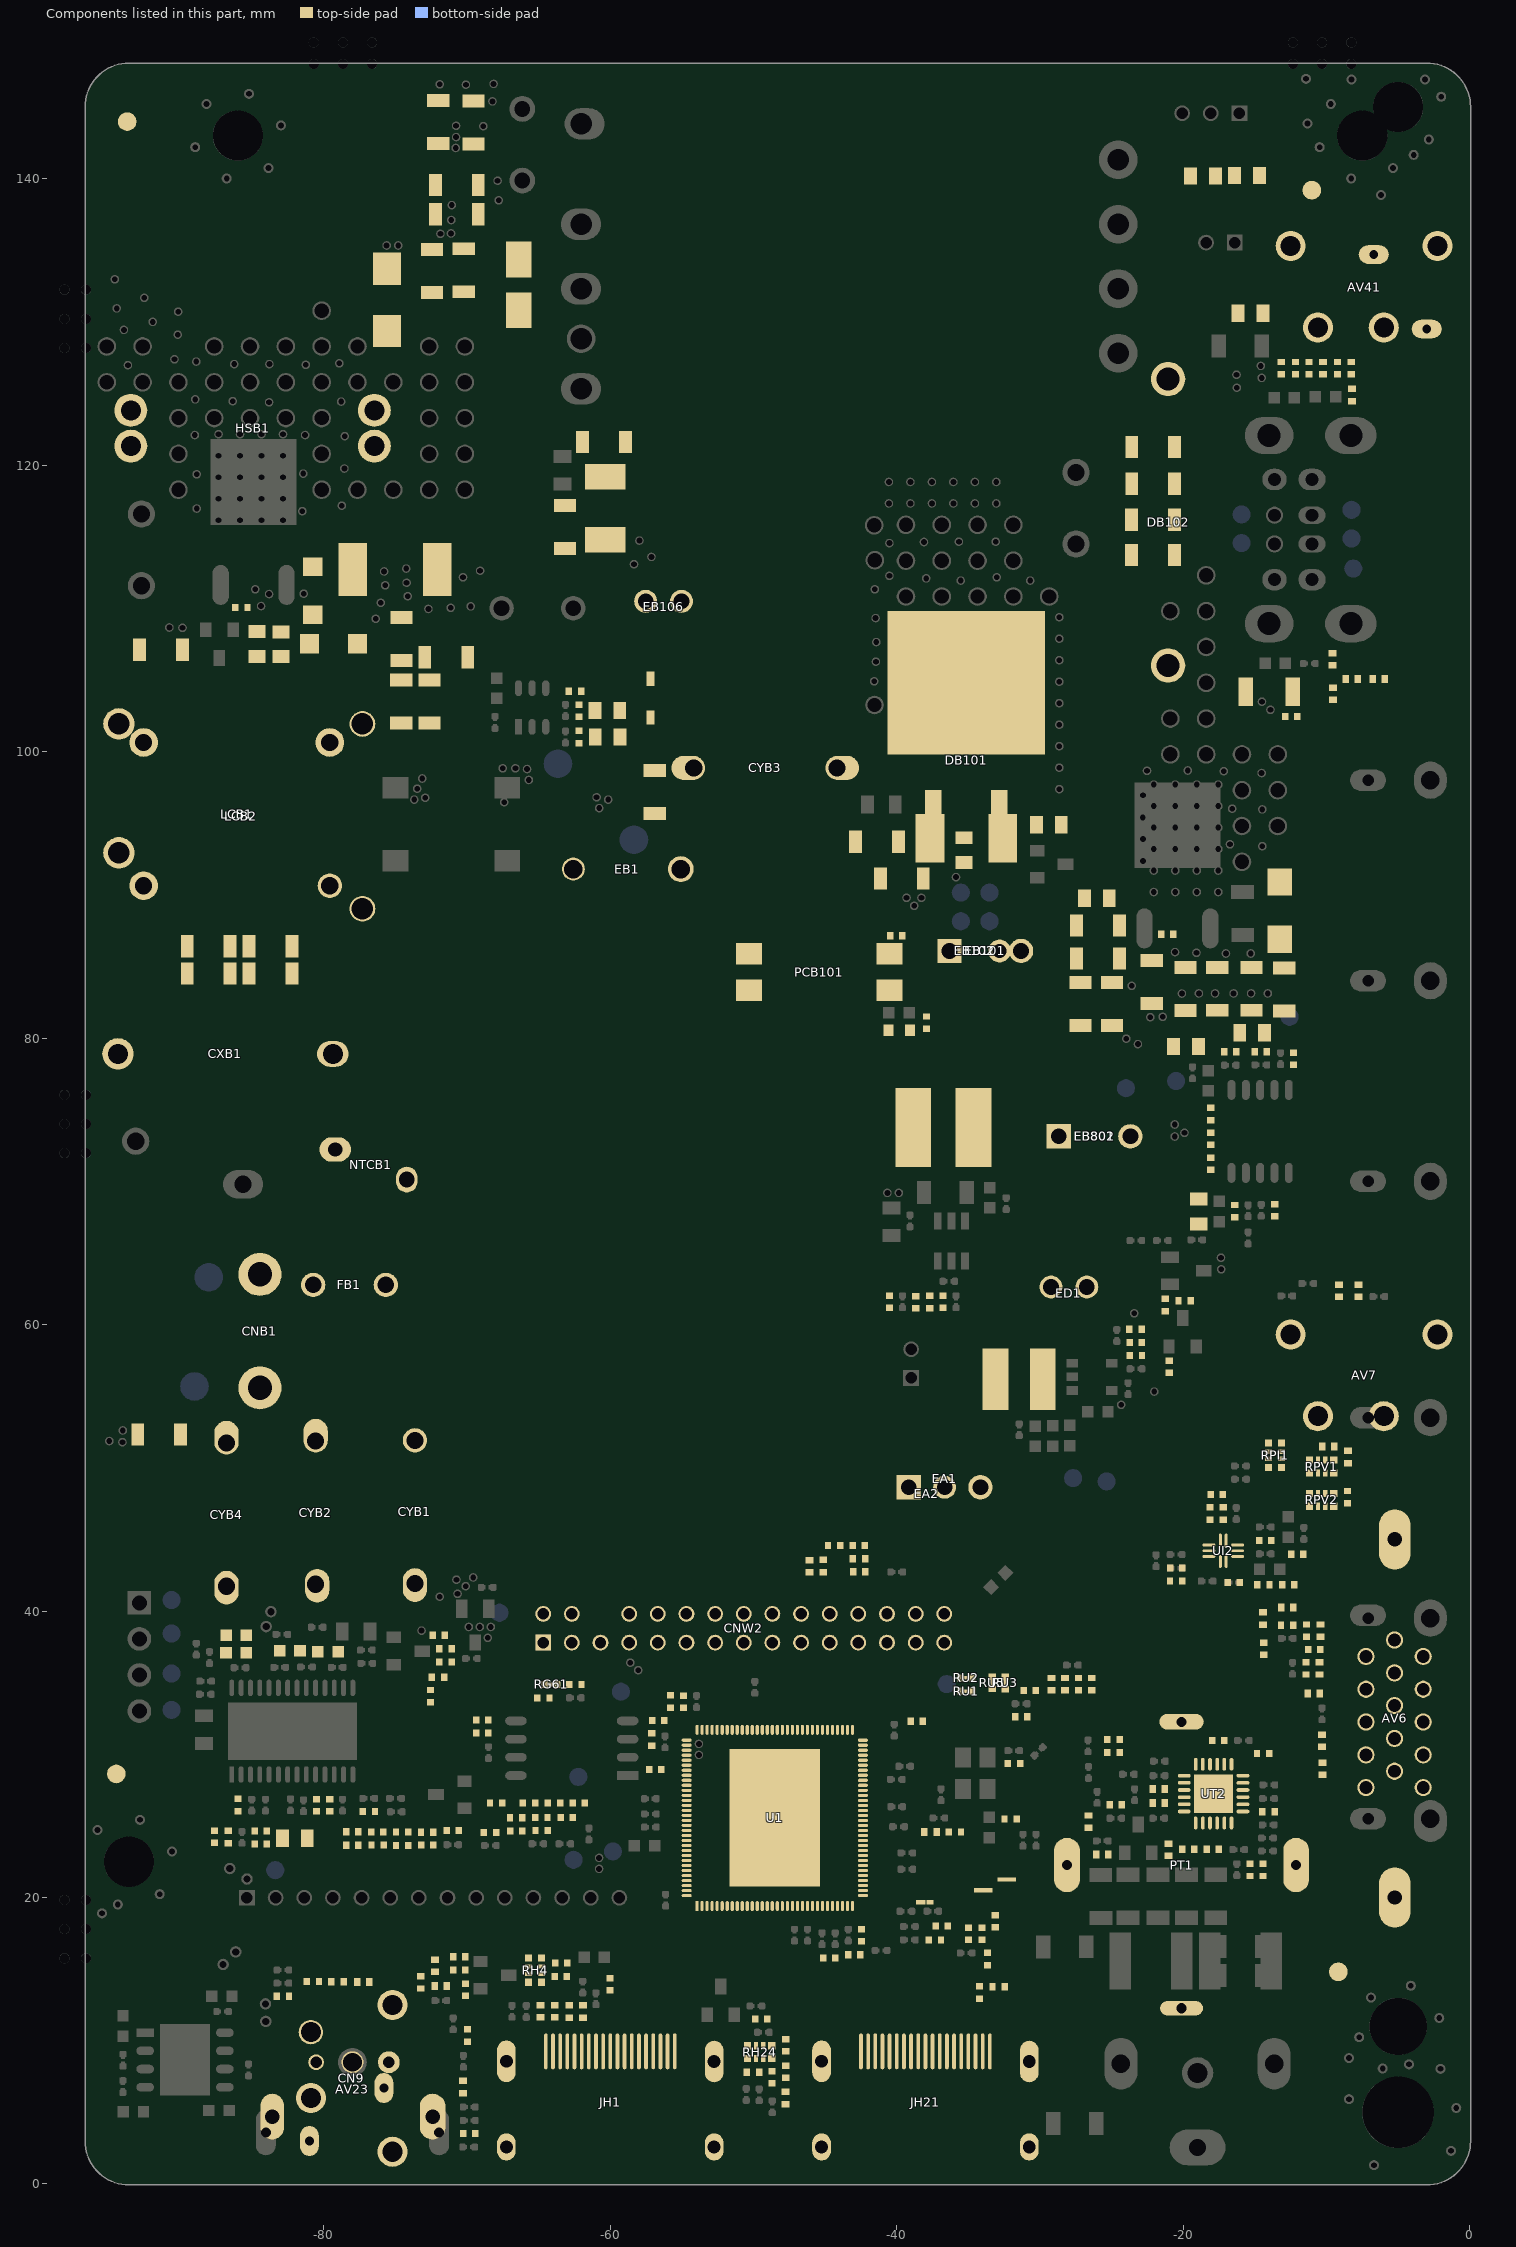
[diagram p0: the components of this part, seen from the top]
# Altium PCB MISC86372.PcbDoc (part 4 of 16)
Units mm, origin at the board's own origin, x right, y up, seen from the top; angles counter-clockwise.
Board outline 96.73 x 148.13 mm, 2 copper layers (TopLayer, BottomLayer), stack 1.571 mm thick; 578 components, 318 nets, 2702 pads, 836 vias.

## Footprints (in the part's own frame and the unit in brackets; to place one, negate y for a bottom-side part, rotate by r counter-clockwise, add the part's x,y. Pads: shape width x height; smd on the part's side, far side on the other; paste and mask are expansions set on the pad) (continued)
CAP13*5-V-10-1#1 [mm] "Walsin;YU1AH471M060DAMD0H;160718（18.03.15  更新孔径）"
  round 1.7 hole 1.2: 1(-5,0)
  oval 2.35x1.7 hole 1.2 copper offset 0.1,0: 2(5,0)
  oval 2.55x1.9 on Top Overlay: 61(-5,0) 61(5,0)
  silkscreen extent -5.71,-3 5.81,3
CAP13*5-V-10-1#2 [mm] "Walsin;YU1AH471M060DAMD0H;160718（18.03.15  更新孔径）"
  oval 2.35x1.7 hole 1.2 copper offset -0.375,0: 1(-5,0)
  oval 2.35x1.7 hole 1.2 copper offset 0.1,0.1: 2(5,0)
  oval 2.55x1.9 on Top Overlay: 61(-5,0) 61(5,0)
  silkscreen extent -5.71,-3 5.81,3
CAP13*5-V-10-1#3 [mm] "Walsin;YU1AH471M060DAMD0H;160718（18.03.15  更新孔径）"
  oval 2.35x1.7 hole 1.2 copper offset -0.375,0: 1(-5,0)
  oval 2.35x1.7 hole 1.2 copper offset 0.375,0: 2(5,0)
  oval 2.55x1.9 on Top Overlay: 61(-5,0) 61(5,0)
  silkscreen extent -5.71,-3 5.81,3
CAP13*5-V-10-1#4 [mm] "Walsin;YU1AH471M060DAMD0H;160718（18.03.15  更新孔径）"
  oval 2.35x1.7 hole 1.2 copper offset -0.375,0: 1(-5,0)
  oval 2.35x1.7 hole 1.2 copper offset 0.1,0: 2(5,0)
  oval 2.55x1.9 on Top Overlay: 61(-5,0) 61(5,0)
  silkscreen extent -5.71,-3 5.81,3
CAP18*8.5-V-15 [mm] "PX334K3ID49H200D9R(凯励)(18.01.12更新孔径）(18.07.18 更新丝印框，加了公差）"
  oval 2.2x1.8 hole 1.4: 1(-7.5,0)
  round 2.2 hole 1.4: 2(7.5,0)
  round 2.4 on Top Overlay: 77(7.5,0) 78(-7.5,0)
  silkscreen extent -9.25,-4.45 9.25,4.45
CAUTION [mm]
  silkscreen extent -10.17,-3.72 12.33,4.08
COLD [mm]
CON2-H7.92 [mm] "因物料底部露金属，20170630增加1.8mm安规禁布"
  round 3 / inner round 3 / far side round 4 hole 1.7: 1(0,3.96)
  round 3 / inner round 3 / far side round 4.4 hole 1.7: 3(0,-3.96)
  round 3.2 on Top Overlay: 109(0,3.96) 110(0,-3.96)
  silkscreen extent -12,-5.94 4.23,5.94, body extent -11.46,-6.04 0.56,5.86, height 8.49
"Conformal Coating" [mm] "三防漆虚线框"
  round 0.3 on Mech2: 0(0,0)
CQC [mm]
D2PAK3 [mm] "伟达电子；SFS1006G;增加TO-252兼容；160309"
  oval 2.794x1.143 smd: 1(5.542,-2.2) 3(5.542,2.4)
  rect 2.794x1.143 smd: 1(5.544,-2.2) 3(5.544,2.4)
  rect 3.4x2 smd paste-5 mask-5: 1(7.494,-2.44) 3(7.494,2.64)
  rect 10x11 smd paste-11 mask-11: 2(-3.356,0.1)
  rect 6x6 smd paste-10 mask-11: 2(-2.158,0.1)
  TopLayer pour cut-out: 3.373,2.4 6.497,2.4 6.497,-2.245 6.438,-2.54 6.271,-2.791 6.02,-2.958 5.725,-3.017 5.725,-3.017 5.725,-2.199 4.141,-2.199 4.141,-3.024 3.847,-2.966 3.598,-2.799 3.432,-2.55 3.373,-2.256 3.373,-2.256
  silkscreen extent -9.13,-5.69 4.84,5.89, body extent -6.91,-5.15 8.79,5.35, height 4.7
D3-H-20 [mm] "肖特基二极管"
  round 2.6 on Top Overlay: 0(10,0) 1(-10,0)
  round 2.4 hole 1.6: A(-10,0) K(10,0)
  silkscreen extent -13,-2.6 13,2.6, body extent -12.62,-2.69 12.63,2.69, height 11.81
DB15-HF-1 [mm] "兴万联电子：WLHD-051A"
  oval 4.4x2.4 on Top Overlay: 0(-12.5,5.227) 0(12.5,5.227)
  round 1.2 hole 0.9: 1(4.33,7.247) 2(2.04,7.247) 3(-0.25,7.247) 4(-2.54,7.247) 5(-4.83,7.247) 6(5.475,5.247) 7(3.185,5.247) 8(0.895,5.247) 9(-1.395,5.247) 10(-3.685,5.247) 11(4.33,3.247) 12(2.04,3.247) 13(-0.25,3.247) 14(-2.54,3.247) 15(-4.83,3.247)
  oval 4.2x2.2 hole 1 slot 3 at 0 deg: 16(-12.5,5.227) 17(12.5,5.227)
  round 1.5 on Top Overlay: 30(-4.83,3.247) 31(-2.54,3.247) 32(-0.25,3.247) 33(2.04,3.247) 34(4.33,3.247) 35(5.475,5.247) 36(3.185,5.247) 37(0.895,5.247) 38(-1.395,5.247) 39(-3.685,5.247) 40(-4.83,7.247) 41(-2.54,7.247) 42(-0.25,7.247) 43(2.04,7.247) 44(4.33,7.247)
  BottomLayer pour cut-out: -4.814,8.609 -4.814,5.885 -4.587,5.885 -4.443,5.742 -3.456,5.742 -3.175,5.461 -3.175,5.029 -3.454,4.75 -4.42,4.75 -4.56,4.609 -4.797,4.609 -4.83,4.576 -4.83,1.885 4.33,1.885 4.33,3.247 4.298,3.279 4.298,4.609 4.105,4.609 3.95,4.764 2.44,4.764 2.285,4.609 1.817,4.609 1.664,4.763 0.648,4.763 0.368,5.042 0.368,5.474 0.622,5.728 1.651,5.728 1.803,5.88 2.286,5.88 2.438,5.728 3.95,5.728 4.107,5.885 4.33,5.885 4.33,8.609
  silkscreen extent -15.59,0 15.59,9.48, body extent -16.75,-62.85 16.75,8.75, height 14.13
DIODE-S0402 [mm] "DVD上使用的ESD"
  rect 0.45x0.55 smd mask+0.051: A(-0.425,0) K(0.425,0)
  silkscreen extent -0.8,-0.43 0.91,0.43, body extent -0.5,-0.25 0.5,0.25, height 0.5
DIODE-S-2 [mm] "1N5819-SMA;170509去除兼容,20180607减少内距0.4mm以兼容SMAF"
  rect 1.8x2.8 smd: A(-2.2,0) K(2.2,0)
  silkscreen extent -3.5,-1.6 3.7,1.61, body extent -2.6,-1.4 2.6,1.4, height 1.91
DIODE-S-12 [mm] "Formosa MS ;BAV19WS THRU BAV21WS/PMEG2010BEA(高度为1.1mm)"
  rect 1x0.55 smd: A(1.35,0) K(-1.35,0)
  silkscreen extent -0.9,-0.67 0.9,0.67, body extent -1.35,-0.63 1.35,0.63, height 1
DIODE-S-14 [mm] "ROHM;FSL14"
  rect 1.3x1.35 smd: A(1.675,0) K(-1.675,0)
  silkscreen extent -1.55,-1 1.55,1, body extent -1.95,-1 1.95,1, height 1.08
DIODE-SMA-1 [mm] "SUF103A(SECOS);14.06.13"
  rect 1.9x1.7 smd: A(-2,0) K(2,0)
  silkscreen extent -2.3,-1.45 2.3,1.45, body extent -2.64,-1.45 2.64,1.45, height 2.44
DIODE-SMA-2 [mm] "LITE-ON,SMAJ20A,0710_2018"
  rect 2.25x1.95 smd mask+0.051: A(-2.17,0) K(2.17,0)
  silkscreen extent -2.27,-1.46 2.3,1.46, body extent -2.59,-1.46 2.62,1.46, height 2.4
DOLBY-SILK [mm]
  silkscreen extent -0.4,-4.5 36.6,5
EC(5*11)-V-2.5 [mm] "机插2.5间距"
  round 1.8 on Top Overlay: 0(-1.25,0) 0(1.25,0)
  round 0.5 on Keep-Out: 0(0,-0.787)
  round 1.6 hole 1.1: 1(-1.25,0) 2(1.25,0)
  BottomLayer lines w0.6: -1.64,-0.31 -2.806,1.556 ; -1.25,0 -2.806,1.556 ; -0.94,0.39 -2.806,1.556 ; 0.94,-0.39 2.806,-1.556 ; 1.25,0 2.806,-1.556 ; 1.64,0.31 2.806,-1.556
  silkscreen extent -2.75,-2.75 3,2.75, body extent -2.48,-2.52 2.5,2.47, height 12.5
EC(6.3*11)-V-2.5#1 [mm] "机插2.5间距"
  round 0.5 on Keep-Out: 0(0,-0.889)
  round 1.6 hole 1.1: 1(-1.25,0) 2(1.25,0)
  round 1.8 on Top Overlay: 5(1.25,0) 6(-1.25,0)
  BottomLayer lines w0.6: -1.665,-0.275 -1.681,-0.244 -1.691,-0.225 ; -1.25,0 -1.417,0.2 -2.279,1.227 -2.664,1.685 ; -0.907,0.361 -0.952,0.395 ; 0.907,-0.361 2.664,-1.685 ; 1.25,0 2.664,-1.685 ; 1.665,0.275 2.664,-1.685 ; -2.664,1.685 -2.501,1.365 -2.382,1.132 ; -2.664,1.685 -1.159,0.551 -0.969,0.408 -0.952,0.395 ; -2.382,1.132 -2.382,1.132 ; -2.382,1.132 -1.805,0 -1.804,-0.003 -1.691,-0.225 ; -1.691,-0.225 -1.691,-0.225 ; -1.691,-0.225 -1.691,-0.225 ; -1.691,-0.225 -1.691,-0.225 ; -1.691,-0.225 -1.691,-0.225 ; -1.691,-0.225 -1.691,-0.225 ; -1.691,-0.225 -1.691,-0.225 ; -1.691,-0.225 -1.691,-0.225 ; -1.691,-0.225 -1.691,-0.225 ; -0.952,0.395 -0.952,0.395 ; -0.952,0.395 -0.952,0.395 ; -0.952,0.395 -0.952,0.395 ; -0.952,0.395 -0.952,0.395 ; -0.952,0.395 -0.952,0.395
  silkscreen extent -3.17,-3.17 3.51,3.17, body extent -3,-3 2.98,2.99, height 12.5
EC(6.3*11)-V-2.5#2 [mm] "机插2.5间距"
  round 0.5 on Keep-Out: 0(0,-0.889)
  round 1.6 hole 1.1: 1(-1.25,0) 2(1.25,0)
  round 1.8 on Top Overlay: 5(1.25,0) 6(-1.25,0)
  BottomLayer lines w0.6: -1.665,-0.275 -1.691,-0.225 -2.664,1.685 ; -1.25,0 -2.664,1.685 ; -0.907,0.361 -0.952,0.395 ; 0.907,-0.361 2.664,-1.685 ; 1.25,0 2.664,-1.685 ; 1.665,0.275 2.664,-1.685 ; -2.664,1.685 -1.25,0.62 -0.952,0.395 ; -0.952,0.395 -0.952,0.395 ; -0.952,0.395 -0.952,0.395 ; -0.952,0.395 -0.952,0.395
  silkscreen extent -3.17,-3.17 3.51,3.17, body extent -3,-3 2.98,2.99, height 12.5
EC(8*11)-V-3.5 [mm]
  rect 1.6x1.6 hole 1: 1(-1.75,0)
  rect 1.8x1.8 on Top Overlay: 1(-1.75,0)
  round 1.8 on Top Overlay: 1(1.75,0)
  round 1.6 hole 1: 2(1.75,0)
  silkscreen extent -4.25,-4.25 4.45,4.25, body extent -3.98,-3.98 4.01,4.01, height 12.51
EC(10*12)-V-5 [mm] "机插5间距"
  rect 1.9x1.9 on Top Overlay: 0(-2.5,0)
  round 0.5 on Keep-Out: 0(-1.01,1.193)
  round 1.9 on Top Overlay: 0(2.5,0)
  rect 1.7x1.7 hole 1.1: 1(-2.5,0)
  round 1.7 hole 1.1: 2(2.5,0)
  BottomLayer lines w0.6: -2.89,-0.31 -2.92,-0.262 ; -2.5,0 -2.685,0.185 -3.632,1.132 -4.056,1.556 ; -2.19,0.39 -2.219,0.408 -2.238,0.42 ; 2.19,-0.39 2.238,-0.42 4.056,-1.556 ; 2.5,0 4.056,-1.556 ; 2.89,0.31 2.92,0.262 4.056,-1.556 ; -4.056,1.556 -4.056,1.556 ; -4.056,1.556 -4.056,1.556 ; -4.056,1.556 -3.321,0.38 -3.084,0 -3.055,-0.046 -2.931,-0.244 -2.92,-0.262 ; -4.056,1.556 -3.751,1.365 -3.529,1.227 -2.454,0.555 -2.238,0.42 ; -4.056,1.556 -4.056,1.556 ; -2.92,-0.262 -2.92,-0.262 ; -2.92,-0.262 -2.92,-0.262 ; -2.92,-0.262 -2.92,-0.262 ; -2.238,0.42 -2.238,0.42
  silkscreen extent -5.25,-5.25 5.57,5.25, body extent -4.98,-4.99 5.01,4.99, height 12.01
EC(10*12.5)-V-5#1 [mm] "机插5间距"
  round 0.5 on Keep-Out: 0(-0.75,0)
  rect 1.7x1.7 hole 1.1: 1(-2.5,0)
  rect 1.9x1.9 on Top Overlay: 1(-2.5,0)
  round 1.9 on Top Overlay: 1(2.5,0)
  round 1.7 hole 1.1: 2(2.5,0)
  BottomLayer lines w0.6: -2.89,-0.31 -2.92,-0.262 ; -2.5,0 -2.749,0.249 -2.815,0.315 -2.994,0.494 -3.084,0.584 -3.315,0.815 -4.056,1.556 ; -2.19,0.39 -2.238,0.42 ; 2.19,-0.39 2.238,-0.42 ; 2.5,0 2.92,-0.42 4.056,-1.556 ; 2.89,0.31 2.92,0.262 ; -4.056,1.556 -3.977,1.507 -3.315,1.093 -2.863,0.81 -2.749,0.739 -2.672,0.691 -2.606,0.65 -2.528,0.601 ; -4.056,1.556 -3.448,0.584 -3.322,0.381 -3.198,0.183 -3.15,0.106 -3.101,0.028 ; -4.056,1.556 -4.056,1.556 ; -3.101,0.028 -3.101,0.028 ; -3.101,0.028 -2.92,-0.262 ; -2.92,-0.262 -2.92,-0.262 ; -2.92,-0.262 -2.92,-0.262 ; -2.528,0.601 -2.528,0.601 ; -2.528,0.601 -2.528,0.601 ; -2.528,0.601 -2.528,0.601 ; -2.528,0.601 -2.5,0.584 -2.337,0.482 -2.266,0.437 -2.254,0.43 -2.238,0.42 ; -2.238,0.42 -2.238,0.42 ; -2.238,0.42 -2.238,0.42 ; -2.238,0.42 -2.238,0.42 ; -2.238,0.42 -2.238,0.42 ; -2.238,0.42 -2.238,0.42 ; 2.238,-0.42 2.92,-0.846 4.056,-1.556 ; 2.238,-0.42 2.238,-0.42 ; 2.92,0.262 3.084,0 3.964,-1.408 4.056,-1.556 ; 2.92,0.262 2.92,0.262
  silkscreen extent -5.2,-5.21 5.57,5.21, body extent -4.98,-4.99 5.01,4.99, height 14.01
EC(10*12.5)-V-5#2 [mm] "机插5间距"
  round 0.5 on Keep-Out: 0(-0.75,0)
  rect 1.7x1.7 hole 1.1: 1(-2.5,0)
  rect 1.9x1.9 on Top Overlay: 1(-2.5,0)
  round 1.9 on Top Overlay: 1(2.5,0)
  round 1.7 hole 1.1: 2(2.5,0)
  BottomLayer lines w0.6: -2.89,-0.31 -4.056,1.556 ; -2.5,0 -4.056,1.556 ; -2.19,0.39 -4.056,1.556 ; 2.19,-0.39 2.238,-0.42 ; 2.5,0 4.056,-1.556 ; 2.89,0.31 2.92,0.262 ; 2.238,-0.42 2.238,-0.42 ; 2.238,-0.42 4.056,-1.556 ; 2.92,0.262 2.92,0.262 ; 2.92,0.262 3.075,0.014 4.056,-1.556
  silkscreen extent -5.2,-5.21 5.57,5.21, body extent -4.98,-4.99 5.01,4.99, height 14.01
EC(13*13)-V-5 [mm] "KF330M200I130A00LR;14-09-17"
  round 1.7 hole 1: 1(-2.5,0) 2(2.5,0)
  round 1.9 on Top Overlay mask+0.076: 2(-2.5,0) 3(2.5,0)
  silkscreen extent -6.75,-6.75 7.26,6.75, body extent -6.7,-6.72 6.82,6.75, height 14.51
EC(18*31.5)-H-7.5 [mm] "SAMXON  (18*45),板上高度15.235mm;170320更新开槽"
  round 1.8 / inner rect 2.5x2.5 / far side rect 2.5x2.5 hole 1.3: 1(3.75,0)
  round 1.6 / inner round 2.5 / far side round 2.5 hole 1.3: 2(-3.75,0)
  round 2.7 on Top Overlay: 2(-3.75,0)
  rect 2.7x2.7 on Top Overlay: 2(3.75,0)
  KeepOutLayer lines w0.127: -6.75,-39.5 -6.75,-4.5 6.75,-4.5 6.75,-39.5 -6.75,-39.5
  silkscreen extent -9.26,-38.11 9.25,-1.26
EVA(7*7*3) [mm] "7*7*3"
  silkscreen extent -4.5,-4.5 4.5,4.5
Fixed [mm] "麦拉片塑胶固定柱(4.50×6.49mm-尼龙-白色)"
  round 2.5 on Keep-Out: 0(0,0)
  silkscreen extent -1.9,-1.9 1.9,1.9
FUSE1.1A-S [mm] "保险丝：FSMD005-1206(FUZETEC)（兼容1206F8.00A063V 高度0.8mm），18.03.07）"
  rect 1x2 smd: 1(-1.65,0) 2(1.65,0)
  silkscreen extent -2.4,-1.2 2.4,1.2, body extent -1.75,-0.9 1.75,0.9, height 1
"FUSE8.5*4-V-5(T3.15AL 250V~)" [mm] "SMT1315AP/2010T1A250VA1(编带/华德)"
  round 1.7 hole 1.15: 1(2.54,0) 2(-2.54,0)
  round 1.9 on Top Overlay: 4(2.54,0) 5(-2.54,0)
  BottomLayer lines w1: 2.811,0.228 3.977,-1.437 ; 2.54,0 3.977,-1.437 ; 2.312,-0.271 3.977,-1.437 ; -2.312,0.271 -3.977,1.437 ; -2.54,0 -3.977,1.437 ; -2.811,-0.228 -3.977,1.437
  silkscreen extent -4.3,-2.1 4.3,2.1, body extent -4.3,-2.1 4.3,2.1, height 8.5
GND#1 [mm] "导通线"
  rect 0.5x0.3 smd paste-0.45 mask-0.45: JP_1K(-0.32,0)
  rect 0.66x0.3 smd paste-0.45 mask-0.45: JP_2K(0.32,0)
GND#2 [mm] "导通线"
  rect 0.66x0.3 smd paste-0.45 mask-0.45: JP_1K(-0.32,0) JP_2K(0.32,0)
HDMI-HS-1#1 [mm] "浙江和丰   HHF-14B000-2SA。17.09.25更新钢网;171107更新焊盘露铜位置(18.04.19 更新大脚孔径）"
  rect 2.2x3.8 on Top Paste: 0(-7.75,4.18) 0(7.753,4.183)
  rect 2.2x6 on Top Paste: 0(-7.75,9.355) 0(7.75,9.355)
  oval 0.26x2.5 smd: 1(4.5,11.258) 2(4,11.258) 3(3.5,11.258) 4(3,11.258) 5(2.5,11.258) 6(2,11.258) 7(1.5,11.258) 8(1,11.258) 9(0.5,11.258) 10(0,11.258) 11(-0.5,11.258) 12(-1,11.258) 13(-1.5,11.258) 14(-2,11.258) 15(-2.5,11.258) 16(-3,11.258) 17(-3.5,11.258) 18(-4,11.258) 19(-4.5,11.258)
  oval 1.3x2.9 hole 0.9 slot 2.5 at 90 deg mask+0.076: 20(-7.25,10.565) 22(7.25,10.55)
  oval 1.3x1.9 hole 0.9 slot 1.5 at 90 deg mask+0.076: 21(-7.25,4.59) 23(7.25,4.59)
  silkscreen extent -7.5,2 7.5,12.19, body extent -10.25,-57.68 10.25,12.17, height 8.42
HDMI-HS-1#2 [mm] "浙江和丰   HHF-14B000-2SA。17.09.25更新钢网;171107更新焊盘露铜位置(18.04.19 更新大脚孔径）"
  rect 2.2x3.8 on Top Paste: 0(-7.75,4.18)
  rect 2.2x6 on Top Paste: 0(-7.75,9.355)
  rect 2.2x3.81 on Top Paste: 0(7.75,9.355)
  rect 2.2x2.032 on Top Paste: 0(7.753,4.183)
  oval 0.26x2.5 smd: 1(4.5,11.258) 2(4,11.258) 3(3.5,11.258) 4(3,11.258) 5(2.5,11.258) 6(2,11.258) 7(1.5,11.258) 8(1,11.258) 9(0.5,11.258) 10(0,11.258) 11(-0.5,11.258) 12(-1,11.258) 13(-1.5,11.258) 14(-2,11.258) 15(-2.5,11.258) 16(-3,11.258) 17(-3.5,11.258) 18(-4,11.258) 19(-4.5,11.258)
  oval 1.3x2.9 hole 0.9 slot 2.5 at 90 deg mask+0.076: 20(-7.25,10.565) 22(7.25,10.55)
  oval 1.3x1.9 hole 0.9 slot 1.5 at 90 deg mask+0.076: 21(-7.25,4.59) 23(7.25,4.59)
  silkscreen extent -7.5,2 7.5,12.19, body extent -10.25,-57.68 10.25,12.17, height 8.42
"Heat-Shrinkable Tube" [mm] "收缩前壁厚0.3+-0.05，收缩后壁厚0.6+-0.1"
  round 0.3 on Mech2: 0(0,0)
"High Voltage" [mm]
  silkscreen extent -0.53,-1.52 0.43,1.27
HOT [mm]
HS149-YZ [mm] "17.5×14.5×0.5-本色-Cu-LHD, 18.05.17  取代HS038的验证封装"
  round 2.3 hole 1.4: 1(-8.5,1.25) 2(-8.5,-1.25) 3(8.5,-1.25) 4(8.5,1.25)
  BottomLayer region: 7.983,-1.016 8.999,-1.016 8.999,1.016 7.983,1.016
  BottomLayer region: -9.017,-1.016 -8.001,-1.016 -8.001,1.016 -9.017,1.016
  silkscreen extent -8.5,-2.5 8.5,2.5
HS(14*14*6) [mm] "14×14×06-THD;14.10.21"
  silkscreen extent -7.1,-7.1 7.1,10.57
L0402 [mm] "电感"
  rect 0.45x0.55 smd mask+0.076: 1(-0.425,0) 2(0.425,0)
  silkscreen extent -0.8,-0.42 0.8,0.43, body extent -0.5,-0.25 0.5,0.25, height 0.5
L0603 [mm] "片式磁珠、电感、ESD"
  rect 0.813x0.8 smd mask+0.076: 1(-0.706,0) 2(0.706,0)
  silkscreen extent -1.27,-0.55 1.27,0.55, body extent -0.8,-0.4 0.8,0.4, height 0.8
L(4*3*2.55)-S [mm] "贴片磁珠；SMB -302540-K5B- L1;15.02.05（17.12.07更新高度信息）"
  rect 2.5x1.8 smd: 1(-1.775,0) 2(1.775,0)
  silkscreen extent -2.12,-1.6 2.12,1.6, body extent -2.55,-1.6 2.55,1.6, height 2.7
L(4.5*3.5)-S [mm] "SMD4532-6R8M-023"
  rect 1.8x4.3 smd: 1(-1.65,0) 2(1.65,0)
  TopLayer pour cut-out: -0.76,2.15 0.796,2.15 0.796,2.141 0.796,-2.149 -0.756,-2.149 -0.756,-2.15
  silkscreen extent -2.83,-2.44 3.3,2.44
L(5.8*4.5)-S [mm] "APC52A45M4R7\电感\Cailank;170317更新阻焊兼容L(4*3.0)-S"
  rect 2.5x5.5 smd paste-5.5: 1(2.105,0) 2(-2.105,0)
  TopLayer pour cut-out: -0.849,2.746 -0.845,2.75 0.861,2.75 0.861,-2.749 0.861,-2.753 0.859,-2.753 -0.862,-2.753
  silkscreen extent -1.5,-2.9 3.88,2.9, body extent -3.06,-2.65 3.08,2.74, height 4.8
L/LC4/20.5*16-H-17*9(12.9) [mm] "SY-UC15C-L001;共模电感；14-04-28"
  round 2.2 hole 1.5 mask+0.076: 1(-8.5,-2.55) 4(-8.5,6.45)
  round 1.8 / inner round 2.2 / far side round 2.2 hole 1.5 mask+0.076: 2(8.5,-6.45) 3(8.5,6.45)
  round 2.4 on Top Overlay mask+0.076: 5(-8.5,6.45) 6(-8.5,-2.55) 7(8.5,-6.45) 8(8.5,6.45)
  silkscreen extent -10.25,-8 10.25,8, body extent -9.8,-7.6 9.8,8.1, height 13.8
L/UU10.5/10*13-2 [mm] "SYUU10.5-L001(协兴电子) 卡扣在侧面"
  round 2 hole 1.2: 1(5,-6.5) 3(-5,6.5) 4(-5,-6.5)
  round 1.7 / inner round 2 / far side round 2 hole 1.2: 2(5,6.5)
  round 2.2 on Top Overlay: 4(-5,6.5) 4(-5,-6.5) 4(5,6.5) 4(5,-6.5)
  silkscreen extent -8,-9.25 11.5,9.25, body extent -8,-8.5 9.5,8.5, height 13.8
Manufacture_Info [mm]
  round 0.3 on Mech2: 0(0,0)
MARK [mm] "SMD 使用"
  round 1.3 smd paste+0 mask+0.65: 0(0,0)
  TopLayer circle w0.254: c0,0 r1.444
  TopLayer pour cut-out: -1.3,0 -1.201,-0.497 -0.919,-0.919 -0.497,-1.201 0,-1.3 0,-1.3 0.497,-1.201 0.919,-0.919 1.201,-0.497 1.3,0 1.3,0 1.201,0.497 0.919,0.919 0.497,1.201 0,1.3 0,1.3 -0.497,1.201 -0.919,0.919 -1.201,0.497 -1.3,0
Mylar [mm] "180×180×0.4mm-PC-黑色"
NTC(10*5)-V5 [mm] "热敏电阻 SCK152R58MSY  (为勤电子）;161022更新椭圆孔"
  oval 1.5x1.8 hole 1.1: 1(-2.5,1.05)
  oval 1.7x2 on Top Overlay: 2(-2.5,1.05)
  oval 2.2x1.7 hole 1 slot 1.5 at 0 deg: 2(2.5,-1.05)
  oval 2.4x1.9 on Top Overlay: 3(2.5,-1.05)
  silkscreen extent -5.77,-2.5 5.77,2.5, body extent -5.75,-2 5.75,2, height 13.75
OC4-S-1 [mm] "巨路国际；肖特基LTV-817S-TA-B"
  rect 1.5x1.8 smd: 1(-1.27,-4.9) 2(1.27,-4.9) 3(1.27,4.9) 4(-1.27,4.9)
  silkscreen extent -2.55,-6.78 2.55,3.5, body extent -2.3,-5.08 2.3,5.08, height 3.88
OPTICAL-HD-3 [mm] "强生GQ-03-08  通用封装 (TR）  塑胶整体高度11.6mm，中心高度6mm(17.04.28,增加丝印宽度到12.3mm）"
  oval 2x3.4 on Top Overlay: 0(-5.6,4.7) 0(5.6,4.7)
  round 1.778 on Top Overlay: 0(-2.54,8.5) 0(0,8.5) 0(2.54,8.5)
  round 1.1 hole 0.8: 1(-2.54,8.5)
  round 1.524 hole 0.8: 2(0,8.5) 3(2.54,8.5)
  oval 1.651x3.2 / inner oval 1.8x3.2 / far side oval 1.8x3.2 hole 1 slot 2.4 at 90 deg: 4(-5.6,4.7)
  oval 1.8x3.2 hole 1 slot 2.4 at 90 deg: 5(5.6,4.7)
  silkscreen extent -6.15,0 6.15,11.8
PCB_NAME [mm]
  round 0.3 on Mech2: 0(0,0)
PCB_TIME [mm]
  round 0.3 on Mech2: 0(0,0)
PHONE-HD-41 [mm] "宇球；PJ7723-F03L3BE-C;160401(17.07.18,孔内边增加0.1mm，外距不变）/（18.03.13更新孔距）"
  round 2.1 hole 1.4: 1(2.8,2.25) 3(2.8,12.5) 4(-2.9,6) 5(-2.9,10.6)
  round 2.3 on Top Overlay: 5(-2.9,10.6) 5(-2.9,6) 6(2.8,2.25) 7(2.8,12.5)
  silkscreen extent -3.65,0 3.65,13.15, body extent -5.05,-62.21 5.05,13, height 12.05
PHONE-HD-42#1 [mm] "YUQIU;PJ7724-F05L3BE-D;160401(17.07.18,孔内边增加0.1mm，外距不变）(18.03.13 更新孔径）"
  oval 1.5x2.3 on Top Overlay: 0(-3,3) 8(2.2,6.7)
  round 2.3 on Top Overlay: 0(-2.9,10.6) 0(-2.9,6) 0(2.8,12.5) 0(2.8,2.25)
  round 2.1 hole 1.4: 1(2.8,2.25) 3(2.8,12.5) 4(-2.9,6) 5(-2.9,10.6)
  oval 1.3x2.1 hole 0.6 slot 1.4 at 90 deg: 2(-3,3) 6(2.2,6.7)
  silkscreen extent -3.65,0 3.65,13.15, body extent -5.05,-62.22 5.05,13, height 12.05
PHONE-HD-42#2 [mm] "YUQIU;PJ7724-F05L3BE-D;160401(17.07.18,孔内边增加0.1mm，外距不变）(18.03.13 更新孔径）"
  oval 1.5x2.3 on Top Overlay: 0(-3,3) 8(2.2,6.7)
  round 2.3 on Top Overlay: 0(-2.9,6) 0(-2.9,10.6) 0(2.8,2.25) 0(2.8,12.5)
  round 2.1 hole 1.4: 1(2.8,2.25) 3(2.8,12.5) 4(-2.9,6)
  oval 1.3x2.1 hole 0.6 slot 1.4 at 90 deg: 2(-3,3) 6(2.2,6.7)
  round 1.7 hole 1.4: 5(-2.9,10.6)
  silkscreen extent -3.65,0 3.65,13.15, body extent -5.05,-62.22 5.05,13, height 12.05
QFN10/0.4 [mm] "Amazing; AZAW2213F"
  oval 1x0.2 smd: 1(-0.7,0.2)
  oval 0.9x0.2 smd: 2(-0.75,-0.2) 6(0.75,-0.2) 7(0.75,0.2)
  oval 0.2x0.9 smd: 3(-0.4,-1) 4(0,-1) 5(0.4,-1) 8(0.4,1) 9(0,1) 10(-0.4,1)
  silkscreen extent -1.58,-0.92 0.72,1.26, body extent -0.7,-0.9 0.7,0.9, height 0.6
QFN24/0.5-3 [mm] "R620D(Rafael Micro)，修改EPAD焊盘/CY8C4014LQI-422(0.6mm)"
  oval 0.9x0.26 smd: 1(-2.05,1.25) 2(-2.05,0.75) 3(-2.05,0.25) 4(-2.05,-0.25) 5(-2.05,-0.75) 6(-2.05,-1.25) 13(2.05,-1.25) 14(2.05,-0.75) 15(2.05,-0.25) 16(2.05,0.25) 17(2.05,0.75) 18(2.05,1.25)
  oval 0.26x0.9 smd: 7(-1.25,-2.05) 8(-0.75,-2.05) 9(-0.25,-2.05) 10(0.25,-2.05) 11(0.75,-2.05) 12(1.25,-2.05) 19(1.25,2.05) 20(0.75,2.05) 21(0.25,2.05) 22(-0.25,2.05) 23(-0.75,2.05) 24(-1.25,2.05)
  rect 2.7x2.7 smd paste-2 mask-2: 25(0,0)
  silkscreen extent -3.38,-3.33 3.21,3.35, body extent -2.08,-2.07 2.07,2.07, height 1
QFN128/0.35-1-9 [mm] "Mstar,TSUMV53RWUT-Z1,18.11.16(19.03.30   减少外延焊盘长度）"
  oct 3x1.9 on Top Paste paste-1: 0(-3.302,-2.21) 0(-3.302,0) 0(-3.302,2.21) 0(0,2.21) 0(0,0) 0(0,-2.21) 0(3.302,-2.21) 0(3.302,0) 0(3.302,2.21)
  oct 3x1.9 on Top Solder paste-1: 0(-3.302,-2.21) 0(-3.302,0) 0(-3.302,2.21) 0(0,2.21) 0(0,0) 0(0,-2.21) 0(3.302,-2.21) 0(3.302,0) 0(3.302,2.21)
  rect 0.7x0.22 smd paste-0.02 mask-0.035: 1(-6.151,5.425)
  oval 0.7x0.22 smd paste-0.02 mask-0.035: 2(-6.151,5.075) 3(-6.151,4.725) 4(-6.151,4.375) 5(-6.151,4.025) 6(-6.151,3.675) 7(-6.151,3.325) 8(-6.151,2.975) 9(-6.151,2.625) 10(-6.151,2.275) 11(-6.151,1.925) 12(-6.151,1.575) 13(-6.151,1.225) 14(-6.151,0.875) 15(-6.151,0.525) 16(-6.151,0.175) 17(-6.151,-0.175) 18(-6.151,-0.525) 19(-6.151,-0.875) 20(-6.151,-1.225) 21(-6.151,-1.575) 22(-6.151,-1.925) 23(-6.151,-2.275) 24(-6.151,-2.625) 25(-6.151,-2.975) 26(-6.151,-3.325) 27(-6.151,-3.675) 28(-6.151,-4.025) 29(-6.151,-4.375) 30(-6.151,-4.725) 31(-6.151,-5.075) 32(-6.151,-5.425) 65(6.151,-5.425) 66(6.151,-5.075) 67(6.151,-4.725) 68(6.151,-4.375) 69(6.151,-4.025) 70(6.151,-3.675) 71(6.151,-3.325) 72(6.151,-2.975) 73(6.151,-2.625) 74(6.151,-2.275) 75(6.151,-1.925) 76(6.151,-1.575) 77(6.151,-1.225) 78(6.151,-0.875) 79(6.151,-0.525) 80(6.151,-0.175) 81(6.151,0.175) 82(6.151,0.525) 83(6.151,0.875) 84(6.151,1.225) 85(6.151,1.575) 86(6.151,1.925) 87(6.151,2.275) 88(6.151,2.625) 89(6.151,2.975) 90(6.151,3.325) 91(6.151,3.675) 92(6.151,4.025) 93(6.151,4.375) 94(6.151,4.725) 95(6.151,5.075) 96(6.151,5.425)
  oval 0.22x0.7 smd paste-0.02 mask-0.035: 33(-5.425,-6.151) 34(-5.075,-6.151) 35(-4.725,-6.151) 36(-4.375,-6.151) 37(-4.025,-6.151) 38(-3.675,-6.151) 39(-3.325,-6.151) 40(-2.975,-6.151) 41(-2.625,-6.151) 42(-2.275,-6.151) 43(-1.925,-6.151) 44(-1.575,-6.151) 45(-1.225,-6.151) 46(-0.875,-6.151) 47(-0.525,-6.151) 48(-0.175,-6.151) 49(0.175,-6.151) 50(0.525,-6.151) 51(0.875,-6.151) 52(1.225,-6.151) 53(1.575,-6.151) 54(1.925,-6.151) 55(2.275,-6.151) 56(2.625,-6.151) 57(2.975,-6.151) 58(3.325,-6.151) 59(3.675,-6.151) 60(4.025,-6.151) 61(4.375,-6.151) 62(4.725,-6.151) 63(5.075,-6.151) 64(5.425,-6.151) 97(5.425,6.151) 98(5.075,6.151) 99(4.725,6.151) 100(4.375,6.151) 101(4.025,6.151) 102(3.675,6.151) 103(3.325,6.151) 104(2.975,6.151) 105(2.625,6.151) 106(2.275,6.151) 107(1.925,6.151) 108(1.575,6.151) 109(1.225,6.151) 110(0.875,6.151) 111(0.525,6.151) 112(0.175,6.151) 113(-0.175,6.151) 114(-0.525,6.151) 115(-0.875,6.151) 116(-1.225,6.151) 117(-1.575,6.151) 118(-1.925,6.151) 119(-2.275,6.151) 120(-2.625,6.151) 121(-2.975,6.151) 122(-3.325,6.151) 123(-3.675,6.151) 124(-4.025,6.151) 125(-4.375,6.151) 126(-4.725,6.151) 127(-5.075,6.151) 128(-5.425,6.151)
  rect 9.6x6.3 smd paste-6 mask-6: EPAD(0,0)
  silkscreen extent -7.48,-7.42 7.42,7.4, body extent -6.2,-6.2 6.2,6.2, height 0.95
R0402 [mm] "片式电阻"
  rect 0.45x0.5 smd mask+0.076: 1(-0.425,0) 2(0.425,0)
  silkscreen extent -0.8,-0.4 0.8,0.4, body extent -0.5,-0.25 0.5,0.25, height 0.5
R0402SC [mm]
  rect 0.45x0.5 smd mask+0.076: 1(-0.425,0) 2(0.425,0)
  rect 0.42x0.25 smd paste-0.5 mask-0.5: 3(0,0)
  silkscreen extent -0.8,-0.4 0.8,0.4, body extent -0.5,-0.25 0.5,0.25, height 0.5
R0603 [mm] "贴片电阻"
  rect 0.7x0.8 smd mask+0.076: 1(-0.756,0) 2(0.756,0)
  silkscreen extent -1.25,-0.54 1.25,0.54, body extent -0.8,-0.4 0.8,0.4, height 0.8
R0805 [mm] "贴片电阻"
  rect 0.9x1.2 smd mask+0.076: 1(-0.866,0) 2(0.866,0)
  silkscreen extent -1.47,-0.75 1.47,0.75, body extent -1,-0.62 1,0.63, height 0.5
R1206 [mm] "贴片电阻"
  rect 0.9x1.55 smd mask+0.076: 1(-1.5,0) 2(1.5,0)
  silkscreen extent -2.1,-0.93 2.1,0.93, body extent -1.6,-0.8 1.6,0.8, height 0.55
R2512-1 [mm] "PSA;Size 2512 2W;16.01.20(17.06.19修改焊盘大小，增强爬锡，解决浮高问题）"
  rect 2x3.7 smd: 1(-2.95,0) 2(2.95,0)
  silkscreen extent -3.3,-2 3.3,2, body extent -3.25,-1.65 3.25,1.65, height 0.75
RA0402 [mm] "排阻"
  rect 0.5x0.5 smd mask+0.076: 1(-0.45,0.85) 2(0.45,0.85) 7(-0.45,-0.85) 8(0.45,-0.85)
  rect 0.5x0.3 smd mask+0.076: 3(-0.45,0.25) 4(0.45,0.25) 5(-0.45,-0.25) 6(0.45,-0.25)
  silkscreen extent -0.85,-1.27 0.85,1.27, body extent -0.51,-1 0.51,1, height 0.35
SHIELD(16*20*6) [mm] "屏蔽罩：用于与高频头分离的做法"
  oval 2.1x4.1 on Top Overlay: 0(-8,10) 0(8,10)
  oval 4.1x2.1 on Top Overlay: 0(0,0) 0(0,20)
  oval 3x1 / inner oval 3.8x1.8 / far side oval 3.8x1.8 hole 0.7 slot 2.7 at 0 deg: 1(0,0)
  oval 1.8x3.8 hole 0.7 slot 2.7 at 90 deg: 2(8,10) 4(-8,10)
  oval 3.1x1.1 / inner oval 3.8x1.8 / far side oval 3.8x1.8 hole 0.7 slot 2.7 at 0 deg: 3(0,20)
  silkscreen extent -9,-1 9,21, body extent -8.57,-0.15 8.57,20.15, height 6
"Silica gel-15" [mm] "硅胶"
  silkscreen extent -3,-7.5 3,7.5
SIP2*15/2.0D-2 [mm] "捷仕泰-XXXXXXXXXXX 12106专用，缺第六脚/LK-HEPHM20012150-006"
  round 1.3 on Top Overlay: 0(-14,-1) 0(-14,1) 0(-12,-1) 0(-12,1) 0(-10,-1) 0(-10,1) 0(-8,-1) 0(-8,1) 0(-6,-1) 0(-6,1) 0(-4,-1) 0(-4,1) 0(-2,-1) 0(-2,1) 0(0,-1) 0(0,1) 0(2,-1) 0(2,1) 0(4,-1) 0(4,1) 0(6,-1) 0(6,1) 0(8,-1) 0(8,1) 0(10,1) 0(12,-1) 0(12,1) 0(14,-1)
  round 1.3 on Bottom Solder: 0(10,-1)
  rect 1.3x1.3 on Top Overlay: 0(14,1)
  rect 1.1x1.1 hole 0.8: 1(14,1)
  round 1.1 hole 0.8: 2(14,-1) 3(12,1) 4(12,-1) 5(10,1) 7(8,1) 8(8,-1) 9(6,1) 10(6,-1) 11(4,1) 12(4,-1) 13(2,1) 14(2,-1) 15(0,1) 16(0,-1) 17(-2,1) 18(-2,-1) 19(-4,1) 20(-4,-1) 21(-6,1) 22(-6,-1) 23(-8,1) 24(-8,-1) 25(-10,1) 26(-10,-1) 27(-12,1) 28(-12,-1) 29(-14,1) 30(-14,-1)
  silkscreen extent -15.1,-3 15.65,3, body extent -15,-2.1 15,2.1, height 6